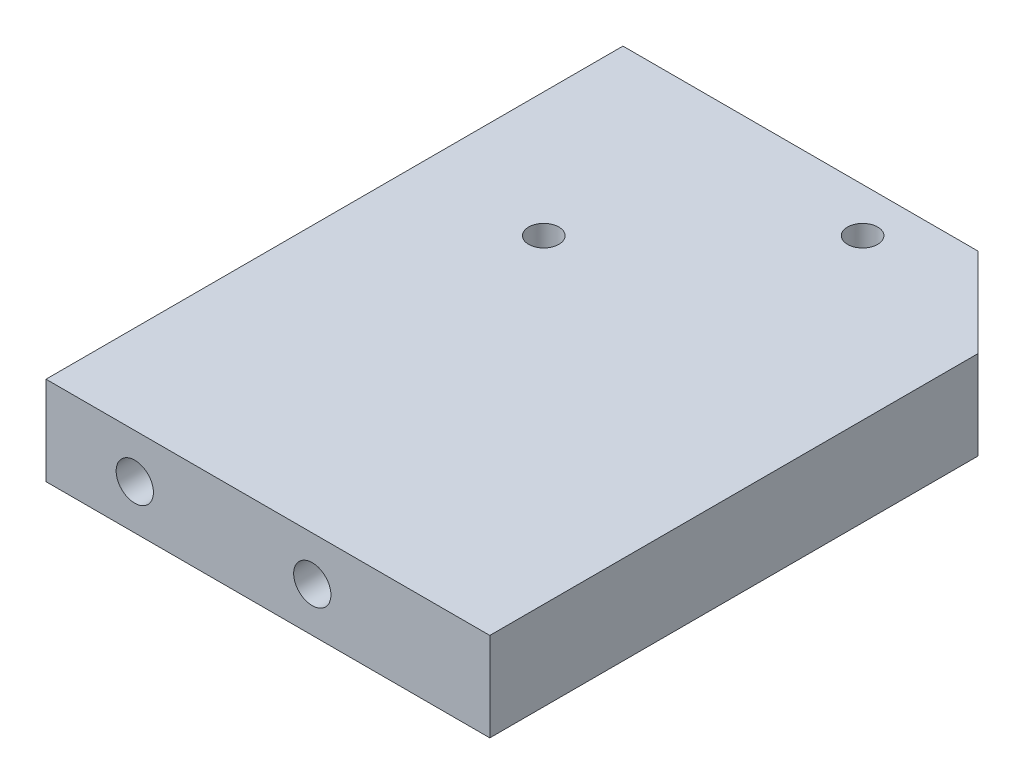
from build123d import *

# Parameters (mm, degrees)
SKETCH_1_W                   = 50
SKETCH_1_H                   = 65
EXTRUDE_1_DEPTH              = 5
CHAMFER_1_SIZE               = 10
HOLE_WIZARD_M5_1_D           = 4.2
HOLE_WIZARD_M5_1_DEPTH       = 12.4
HOLE_WIZARD_M5_1_TIP         = 1.2618073
HOLE_WIZARD_M3_1_D           = 3.4
HOLE_WIZARD_M3_1_CBORE_D     = 6.5
HOLE_WIZARD_M3_1_CBORE_DEPTH = 3.4
HOLE_WIZARD_M5_2_D           = 4.2
HOLE_WIZARD_M5_2_DEPTH       = 12.4
HOLE_WIZARD_M5_2_TIP         = 1.2618073


with BuildPart() as part:
    # 草图1 → 凸台-拉伸1 (new, symmetric)
    with BuildSketch(Plane(origin=(0, 0, 0), x_dir=(1, 0, 0), z_dir=(0, 1, 0))):
        Rectangle(SKETCH_1_W, SKETCH_1_H)
    extrude(amount=EXTRUDE_1_DEPTH, both=True)

    # 倒角1
    chamfer_1_edges = [part.edges().sort_by_distance(p)[0] for p in [
        (25, 0, -32.5),
    ]]
    chamfer(chamfer_1_edges, length=CHAMFER_1_SIZE)

    # M5 螺纹孔1
    with Locations(Plane.ZY.offset(25)):
        with Locations((-12.5, 0), (12.5, 0)):
            Hole(HOLE_WIZARD_M5_1_D / 2, depth=HOLE_WIZARD_M5_1_DEPTH)
            with Locations((0, 0, -(HOLE_WIZARD_M5_1_DEPTH + HOLE_WIZARD_M5_1_TIP / 2))):  # 118° drill point
                Cone(0, HOLE_WIZARD_M5_1_D / 2, HOLE_WIZARD_M5_1_TIP, mode=Mode.SUBTRACT)

    # M3 六角凹头螺钉的柱形沉头孔1 (through all)
    with Locations(Plane(origin=(0, -5, 0), x_dir=(-1, 0, 0), z_dir=(0, -1, 0))):
        with Locations((-7, 27.5), (10.960512242, 9.539487758)):
            CounterBoreHole(HOLE_WIZARD_M3_1_D / 2, HOLE_WIZARD_M3_1_CBORE_D / 2, HOLE_WIZARD_M3_1_CBORE_DEPTH)

    # M5 螺纹孔2
    with Locations(Plane.XY.offset(32.5)):
        with Locations((-15, 0), (5, 0)):
            Hole(HOLE_WIZARD_M5_2_D / 2, depth=HOLE_WIZARD_M5_2_DEPTH)
            with Locations((0, 0, -(HOLE_WIZARD_M5_2_DEPTH + HOLE_WIZARD_M5_2_TIP / 2))):  # 118° drill point
                Cone(0, HOLE_WIZARD_M5_2_D / 2, HOLE_WIZARD_M5_2_TIP, mode=Mode.SUBTRACT)


solid = part.part
